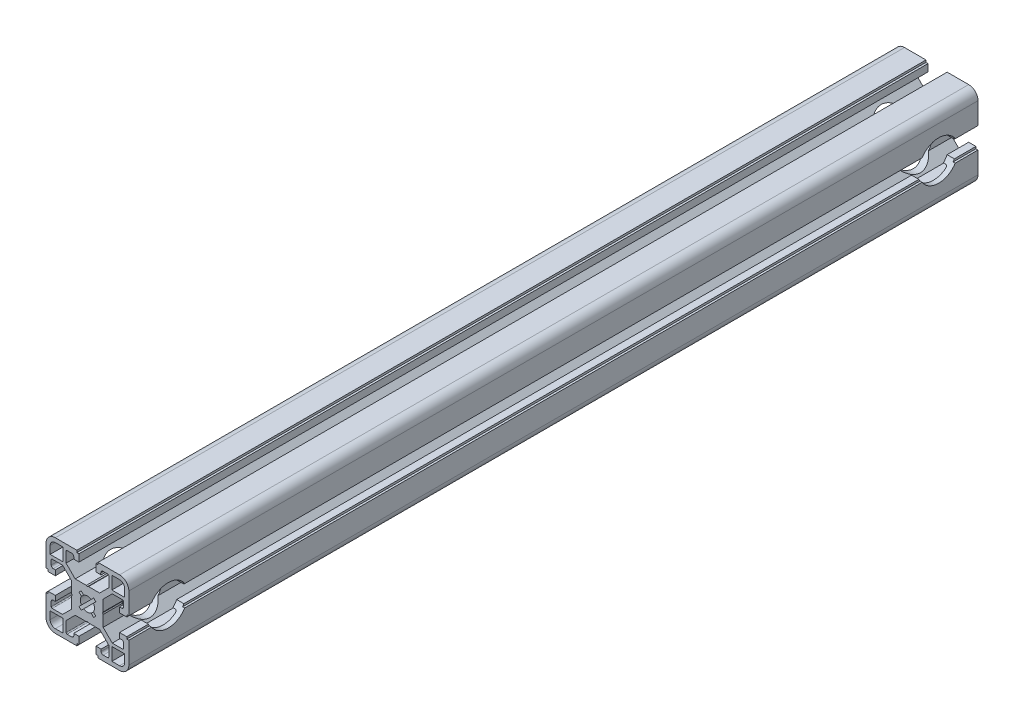
SolidWorks part; units mm, degrees
material "6061 GB/T6892-2006"
ref_plane "前视" through (0, 0, 0) normal (0, 0, 1) x (1, 0, 0)
ref_plane "上视" through (0, 0, 0) normal (0, 1, 0) x (1, 0, 0)
ref_plane "右视" through (0, 0, 0) normal (1, 0, 0) x (0, 0, -1)
sketch "草图1" plane through (0, 0, 0) normal (0, 0, 1) x (1, 0, 0)
  line L0 (-18.9995, -4.1003) -> (-18.9995, -5.1003)
  line L1 (-18.9995, -5.1003) -> (-19.9995, -5.1003)
  line L2 (-19.9995, -5.1003) -> (-19.9995, -15.5003)
  line L3 (-15.4995, -20.0003) -> (-5.0995, -20.0003)
  line L4 (-5.0995, -20.0003) -> (-5.0995, -19.0003)
  line L5 (-5.0995, -19.0003) -> (-4.0995, -19.0003)
  line L6 (-4.0995, -19.0003) -> (-4.0995, -15.5003)
  line L7 (-4.0995, -15.5003) -> (-6.5995, -15.5003)
  line L8 (-6.5995, -15.5003) -> (-6.5995, -16.5003)
  line L9 (-7.5995, -17.5003) -> (-9.7995, -17.5003)
  line L10 (-10.2995, -17.0003) -> (-10.2995, -11.9973)
  line L11 (-10.2995, -11.9973) -> (-5.9025, -7.6003)
  line L12 (-5.9025, -7.6003) -> (-0.5195, -7.6003)
  line L13 (-0.5195, -7.6003) -> (0.0005, -7.3003)
  line L14 (0.0005, -7.3003) -> (0.5195, -7.6003)
  line L15 (0.5195, -7.6003) -> (5.9035, -7.6003)
  line L16 (5.9035, -7.6003) -> (10.3005, -11.9973)
  line L17 (10.3005, -11.9973) -> (10.3005, -17.0003)
  line L18 (9.8005, -17.5003) -> (7.6005, -17.5003)
  line L19 (6.6005, -16.5003) -> (6.6005, -15.5003)
  line L20 (6.6005, -15.5003) -> (4.1005, -15.5003)
  line L21 (4.1005, -15.5003) -> (4.1005, -19.0003)
  line L22 (4.1005, -19.0003) -> (5.1005, -19.0003)
  line L23 (5.1005, -19.0003) -> (5.1005, -20.0003)
  line L24 (5.1005, -20.0003) -> (15.5005, -20.0003)
  line L25 (20.0005, -15.5003) -> (20.0005, -5.1003)
  line L26 (20.0005, -5.1003) -> (19.0005, -5.1003)
  line L27 (19.0005, -5.1003) -> (19.0005, -4.1003)
  line L28 (19.0005, -4.1003) -> (15.5005, -4.1003)
  line L29 (15.5005, -4.1003) -> (15.5005, -6.6003)
  line L30 (15.5005, -6.6003) -> (16.5005, -6.6003)
  line L31 (17.5005, -7.6003) -> (17.5005, -9.8003)
  line L32 (17.0005, -10.3003) -> (11.9975, -10.3003)
  line L33 (11.9975, -10.3003) -> (7.6005, -5.9033)
  line L34 (7.6005, -5.9033) -> (7.6005, -0.5203)
  line L35 (7.6005, -0.5203) -> (7.3005, -0.0003)
  line L36 (7.3005, -0.0003) -> (7.6005, 0.5197)
  line L37 (7.6005, 0.5197) -> (7.6005, 5.9027)
  line L38 (7.6005, 5.9027) -> (11.9975, 10.2997)
  line L39 (11.9975, 10.2997) -> (17.0005, 10.2997)
  line L40 (17.5005, 9.7997) -> (17.5005, 7.5997)
  line L41 (16.5005, 6.5997) -> (15.5005, 6.5997)
  line L42 (15.5005, 6.5997) -> (15.5005, 4.0997)
  line L43 (15.5005, 4.0997) -> (19.0005, 4.0997)
  line L44 (19.0005, 4.0997) -> (19.0005, 5.0997)
  line L45 (19.0005, 5.0997) -> (20.0005, 5.0997)
  line L46 (20.0005, 5.0997) -> (20.0005, 15.4997)
  line L47 (15.5005, 19.9997) -> (5.1005, 19.9997)
  line L48 (5.1005, 19.9997) -> (5.1005, 18.9997)
  line L49 (5.1005, 18.9997) -> (4.1005, 18.9997)
  line L50 (4.1005, 18.9997) -> (4.1005, 15.4997)
  line L51 (4.1005, 15.4997) -> (6.6005, 15.4997)
  line L52 (7.6005, 17.4997) -> (9.8005, 17.4997)
  line L53 (10.3005, 16.9997) -> (10.3005, 11.9967)
  line L54 (10.3005, 11.9967) -> (5.9035, 7.5997)
  line L55 (5.9035, 7.5997) -> (0.5195, 7.5997)
  line L56 (0.5195, 7.5997) -> (0.0005, 7.2997)
  line L57 (0.0005, 7.2997) -> (-0.5195, 7.5997)
  line L58 (-0.5195, 7.5997) -> (-5.9025, 7.5997)
  line L59 (-5.9025, 7.5997) -> (-10.2995, 11.9967)
  line L60 (-10.2995, 11.9967) -> (-10.2995, 16.9997)
  line L61 (-9.7995, 17.4997) -> (-7.5995, 17.4997)
  line L62 (-6.5995, 16.4997) -> (-6.5995, 15.4997)
  line L63 (-6.5995, 15.4997) -> (-4.0995, 15.4997)
  line L64 (-4.0995, 15.4997) -> (-4.0995, 18.9997)
  line L65 (-4.0995, 18.9997) -> (-5.0995, 18.9997)
  line L66 (-5.0995, 18.9997) -> (-5.0995, 19.9997)
  line L67 (-5.0995, 19.9997) -> (-15.4995, 19.9997)
  line L68 (-19.9995, 15.4997) -> (-19.9995, 5.0997)
  line L69 (-19.9995, 5.0997) -> (-18.9995, 5.0997)
  line L70 (-18.9995, 5.0997) -> (-18.9995, 4.0997)
  line L71 (-18.9995, 4.0997) -> (-15.4995, 4.0997)
  line L72 (-15.4995, 4.0997) -> (-15.4995, 6.5997)
  line L73 (-15.4995, 6.5997) -> (-16.4995, 6.5997)
  line L74 (-17.4995, 7.5997) -> (-17.4995, 9.7997)
  line L75 (-16.9995, 10.2997) -> (-11.9965, 10.2997)
  line L76 (-11.9965, 10.2997) -> (-7.5995, 5.9027)
  line L77 (-7.5995, 5.9027) -> (-7.5995, 0.5197)
  line L78 (-7.5995, 0.5197) -> (-7.2995, -0.0003)
  line L79 (-7.2995, -0.0003) -> (-7.5995, -0.5203)
  line L80 (-7.5995, -0.5203) -> (-7.5995, -5.9033)
  line L81 (-7.5995, -5.9033) -> (-11.9965, -10.3003)
  line L82 (-11.9965, -10.3003) -> (-16.9995, -10.3003)
  line L83 (-17.4995, -9.8003) -> (-17.4995, -7.6003)
  line L84 (-16.4995, -6.6003) -> (-15.4995, -6.6003)
  line L85 (-15.4995, -6.6003) -> (-15.4995, -4.1003)
  line L86 (-15.4995, -4.1003) -> (-18.9995, -4.1003)
  line L87 (15.5005, -18.0003) -> (11.8005, -18.0003)
  line L88 (11.8005, -18.0003) -> (11.8005, -11.8003)
  line L89 (11.8005, -11.8003) -> (18.0005, -11.8003)
  line L90 (18.0005, -11.8003) -> (18.0005, -15.5003)
  line L91 (18.0005, 11.7997) -> (11.8005, 11.7997)
  line L92 (11.8005, 11.7997) -> (11.8005, 17.9997)
  line L93 (11.8005, 17.9997) -> (15.5005, 17.9997)
  line L94 (18.0005, 15.4997) -> (18.0005, 11.7997)
  line L95 (-1.8145, -2.8753) -> (-3.0044, -4.0665)
  line L96 (-3.0044, -4.0665) -> (-4.0656, -3.0052)
  line L97 (-4.0656, -3.0052) -> (-2.8745, -1.8153)
  line L98 (-2.8745, 1.8147) -> (-4.0644, 3.0058)
  line L99 (-4.0644, 3.0058) -> (-3.0044, 4.0658)
  line L100 (-3.0044, 4.0658) -> (-1.8145, 2.8747)
  line L101 (1.8145, 2.8747) -> (3.0055, 4.0657)
  line L102 (3.0055, 4.0657) -> (4.0666, 3.0045)
  line L103 (4.0666, 3.0045) -> (2.8755, 1.8147)
  line L104 (2.8755, -1.8153) -> (4.0666, -3.0052)
  line L105 (4.0666, -3.0052) -> (3.0055, -4.0663)
  line L106 (3.0055, -4.0663) -> (1.8145, -2.8753)
  line L107 (-17.9995, -15.5003) -> (-17.9995, -11.8003)
  line L108 (-17.9995, -11.8003) -> (-11.7995, -11.8003)
  line L109 (-11.7995, -11.8003) -> (-11.7995, -18.0003)
  line L110 (-11.7995, -18.0003) -> (-15.4995, -18.0003)
  line L111 (-11.7995, 17.9997) -> (-11.7995, 11.7997)
  line L112 (-11.7995, 11.7997) -> (-17.9995, 11.7997)
  line L113 (-17.9995, 11.7997) -> (-17.9995, 15.4997)
  line L114 (-15.4995, 17.9997) -> (-11.7995, 17.9997)
  arc A0 (-19.9995, -15.5003) -> (-15.4995, -20.0003) centre (-15.4995, -15.5003) ccw
  arc A1 (-6.5995, -16.5003) -> (-7.5995, -17.5003) centre (-7.5995, -16.5003) cw
  arc A2 (-9.7995, -17.5003) -> (-10.2995, -17.0003) centre (-9.7995, -17.0003) cw
  arc A3 (10.3005, -17.0003) -> (9.8005, -17.5003) centre (9.8005, -17.0003) cw
  arc A4 (7.6005, -17.5003) -> (6.6005, -16.5003) centre (7.6005, -16.5003) cw
  arc A5 (15.5005, -20.0003) -> (20.0005, -15.5003) centre (15.5005, -15.5003) ccw
  arc A6 (16.5005, -6.6003) -> (17.5005, -7.6003) centre (16.5005, -7.6003) cw
  arc A7 (17.5005, -9.8003) -> (17.0005, -10.3003) centre (17.0005, -9.8003) cw
  arc A8 (17.0005, 10.2997) -> (17.5005, 9.7997) centre (17.0005, 9.7997) cw
  arc A9 (17.5005, 7.5997) -> (16.5005, 6.5997) centre (16.5005, 7.5997) cw
  arc A10 (20.0005, 15.4997) -> (15.5005, 19.9997) centre (15.5005, 15.4997) ccw
  arc A11 (6.6005, 15.4997) -> (6.6005, 16.4997) centre (7.1003, 15.9997) cw
  arc A12 (6.6005, 16.4997) -> (7.6005, 17.4997) centre (7.6005, 16.4997) cw
  arc A13 (9.8005, 17.4997) -> (10.3005, 16.9997) centre (9.8005, 16.9997) cw
  arc A14 (-10.2995, 16.9997) -> (-9.7995, 17.4997) centre (-9.7995, 16.9997) cw
  arc A15 (-7.5995, 17.4997) -> (-6.5995, 16.4997) centre (-7.5995, 16.4997) cw
  arc A16 (-15.4995, 19.9997) -> (-19.9995, 15.4997) centre (-15.4995, 15.4997) ccw
  arc A17 (-16.4995, 6.5997) -> (-17.4995, 7.5997) centre (-16.4995, 7.5997) cw
  arc A18 (-17.4995, 9.7997) -> (-16.9995, 10.2997) centre (-16.9995, 9.7997) cw
  arc A19 (-16.9995, -10.3003) -> (-17.4995, -9.8003) centre (-16.9995, -9.8003) cw
  arc A20 (-17.4995, -7.6003) -> (-16.4995, -6.6003) centre (-16.4995, -7.6003) cw
  arc A21 (18.0005, -15.5003) -> (15.5005, -18.0003) centre (15.5005, -15.5003) cw
  arc A22 (15.5005, 17.9997) -> (18.0005, 15.4997) centre (15.5005, 15.4997) cw
  arc A23 (-2.8745, -1.8153) -> (-2.8745, 1.8147) centre (0.0005, -0.0003) cw
  arc A24 (-1.8145, 2.8747) -> (1.8145, 2.8747) centre (0, -0.0007) cw
  arc A25 (2.8755, 1.8147) -> (2.8755, -1.8153) centre (0.0005, -0.0003) cw
  arc A26 (1.8145, -2.8753) -> (-1.8145, -2.8753) centre (0, 0) cw
  arc A27 (-15.4995, -18.0003) -> (-17.9995, -15.5003) centre (-15.4995, -15.5003) cw
  arc A28 (-17.9995, 15.4997) -> (-15.4995, 17.9997) centre (-15.4995, 15.4997) cw
extrude "凸台-拉伸1" add sketch "草图1" against normal blind 410
hole_wizard "Ø19.0 (19) 直径孔1" positions "草图2" profile "草图3" hole size "Ø19.0" standard "GB" end condition through all
sketch "草图2" plane through (20.0005, 0, 0) normal (1, 0, 0) x (0, 0, -1)
  line L0 (410, -0.0003) -> (0, -0.0003) construction
  point P0 (19, -0.0003)
  point P4 (391, -0.0003)
  dimension "D1" = 19
  dimension "D2" = 19
sketch "草图3" plane through (20.0005, -0.0003, -19) normal (0, 1, 0) x (0, 0, -1)
  line L0 (0, 0) -> (0, 40)
  line L1 (0, 40) -> (9.5, 40)
  line L2 (9.5, 40) -> (9.5, 0)
  line L5 (9.5, 0) -> (0, 0)
  line L11 (0, -6.35) -> (0, 107.95) construction
  dimension "通孔孔直径" = 19
  dimension "通孔孔深度" = 40
